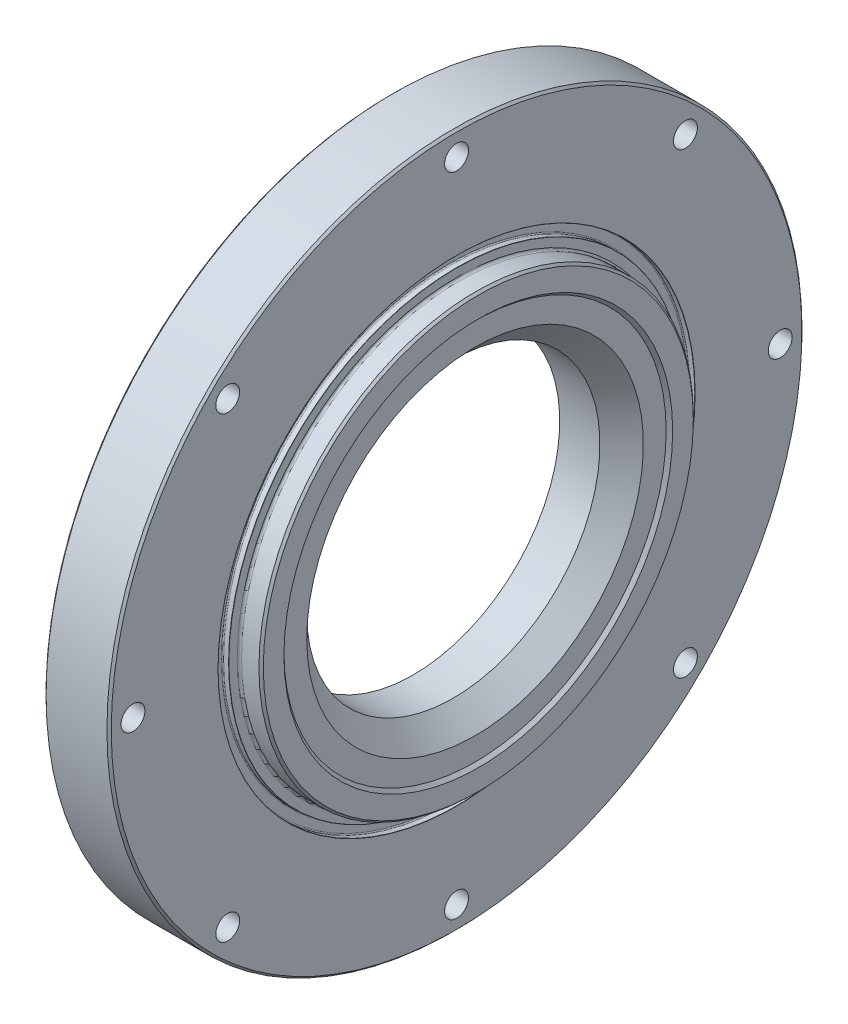
from build123d import *

# Parameters (mm, degrees)
FILLET1_R          = 2
CHAMFER1_SIZE      = 2
FILLET2_R          = 2
CHAMFER2_SIZE      = 2
SKETCH2_R          = 11
CUT_EXTRUDE1_DEPTH = 460.565011723
SKETCH3_R          = 16.5
CUT_EXTRUDE2_DEPTH = 35


with BuildPart() as part:
    # Sketch1 → Revolve1 (revolve)
    with BuildSketch(Plane.XY, mode=Mode.PRIVATE) as revolve1_sk:
        with BuildLine():
            Line((0, 273.05), (0, 320))
            Line((0, 320), (60, 320))
            Line((60, 320), (60, 219.7))
            ThreePointArc((60, 219.7), (59.941421356, 219.558578644), (59.8, 219.5))
            Line((59.8, 219.5), (55.28, 219.5))
            ThreePointArc((55.28, 219.5), (54.572893219, 219.207106781), (54.28, 218.5))
            Line((54.28, 218.5), (54.28, 210.8))
            ThreePointArc((54.28, 210.8), (54.572893219, 210.092893219), (55.28, 209.8))
            Line((55.28, 209.8), (59.8, 209.8))
            ThreePointArc((59.8, 209.8), (59.941421356, 209.741421356), (60, 209.6))
            Line((60, 209.6), (60, 200))
            Line((60, 200), (80, 200))
            Line((80, 200), (80, 179))
            Line((80, 179), (77, 176))
            Line((77, 176), (77, 155))
            Line((77, 155), (57, 135))
            Line((57, 135), (20, 135))
            Line((20, 135), (20, 234.6))
            ThreePointArc((20, 234.6), (20.058578644, 234.741421356), (20.2, 234.8))
            Line((20.2, 234.8), (24.72, 234.8))
            ThreePointArc((24.72, 234.8), (25.427106781, 235.092893219), (25.72, 235.8))
            Line((25.72, 235.8), (25.72, 243.5))
            ThreePointArc((25.72, 243.5), (25.427106781, 244.207106781), (24.72, 244.5))
            Line((24.72, 244.5), (20.2, 244.5))
            ThreePointArc((20.2, 244.5), (20.058578644, 244.558578644), (20, 244.7))
            Line((20, 244.7), (20, 273.05))
            Line((20, 273.05), (0, 273.05))
        make_face()
    revolve(revolve1_sk.sketch.rotate(Axis((0, 0, 0), (1, 0, 0)), 90), axis=Axis((0, 0, 0), (1, 0, 0)))

    # Fillet1
    fillet1_edges = [part.edges().sort_by_distance(p)[0] for p in [
        (20, 0, -273.05),
    ]]
    fillet(fillet1_edges, radius=FILLET1_R)

    # Chamfer1
    chamfer1_edges = [part.edges().sort_by_distance(p)[0] for p in [
        (0, 0, -273.05),
        (0, 0, -320),
        (60, 0, -320),
    ]]
    chamfer(chamfer1_edges, length=CHAMFER1_SIZE)

    # Fillet2
    fillet2_edges = [part.edges().sort_by_distance(p)[0] for p in [
        (60, 0, -200),
    ]]
    fillet(fillet2_edges, radius=FILLET2_R)

    # Chamfer2
    chamfer2_edges = [part.edges().sort_by_distance(p)[0] for p in [
        (80, 0, -200),
    ]]
    chamfer(chamfer2_edges, length=CHAMFER2_SIZE)

    # Sketch2 → Cut-Extrude1 (cut, through all)
    with BuildSketch(Plane.ZY):
        with Locations((0, 298)):
            Circle(SKETCH2_R)
        with Locations((210.717820794, 210.717820794)):
            Circle(SKETCH2_R)
        with Locations((298, 0)):
            Circle(SKETCH2_R)
        with Locations((210.717820794, -210.717820794)):
            Circle(SKETCH2_R)
        with Locations((0, -298)):
            Circle(SKETCH2_R)
        with Locations((-210.717820794, -210.717820794)):
            Circle(SKETCH2_R)
        with Locations((-298, 0)):
            Circle(SKETCH2_R)
        with Locations((-210.717820794, 210.717820794)):
            Circle(SKETCH2_R)
    extrude(amount=-CUT_EXTRUDE1_DEPTH, mode=Mode.SUBTRACT)

    # Sketch3 → Cut-Extrude2 (cut)
    with BuildSketch(Plane.ZY):
        with Locations((0, 298)):
            Circle(SKETCH3_R)
        with Locations((210.717820794, 210.717820794)):
            Circle(SKETCH3_R)
        with Locations((298, 0)):
            Circle(SKETCH3_R)
        with Locations((210.717820794, -210.717820794)):
            Circle(SKETCH3_R)
        with Locations((0, -298)):
            Circle(SKETCH3_R)
        with Locations((-210.717820794, -210.717820794)):
            Circle(SKETCH3_R)
        with Locations((-298, 0)):
            Circle(SKETCH3_R)
        with Locations((-210.717820794, 210.717820794)):
            Circle(SKETCH3_R)
    extrude(amount=-CUT_EXTRUDE2_DEPTH, mode=Mode.SUBTRACT)


solid = part.part
